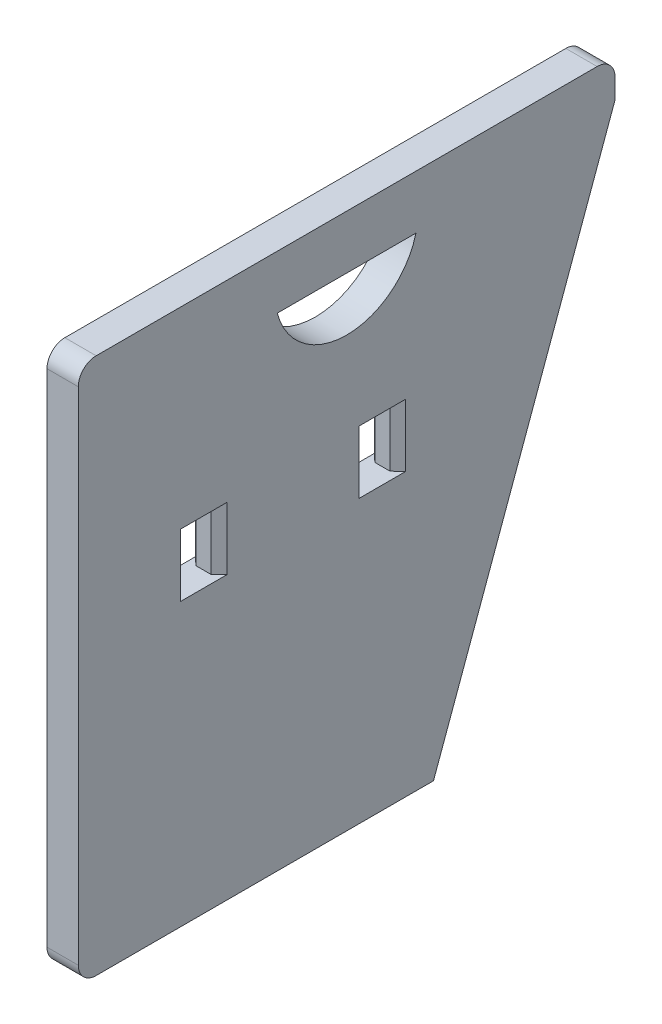
SolidWorks part; units mm, degrees
material "Q235-A"
ref_plane "Front Plane" through (0, 0, 0) normal (0, 0, 1) x (1, 0, 0)
ref_plane "Top Plane" through (0, 0, 0) normal (0, 1, 0) x (1, 0, 0)
ref_plane "Right Plane" through (0, 0, 0) normal (1, 0, 0) x (0, 0, -1)
sketch "Sketch1" plane through (0, 0, 0) normal (1, 0, 0) x (0, 0, -1)
  line L0 (0, 0) -> (0, 300)
  line L1 (0, 300) -> (600, 300)
  line L2 (600, 300) -> (600, 213.7783)
  line L3 (413, -300) -> (0, -300)
  line L4 (0, -300) -> (0, 0)
  line L5 (600, 213.7783) -> (413, -300)
  line L6 (222.5403, 240) -> (377.4597, 240)
  line L7 (0, 0) -> (273.4876, 0) construction
  arc A0 (222.5403, 240) -> (377.4597, 240) centre (300, 260) ccw
  dimension "D1" = 80
  dimension "D2" = 20
  dimension "D3" = 300
  dimension "D4" = 60
  dimension "D5" = 600
  dimension "D6" = 600
  dimension "D7" = 413
  dimension "D8" = 20
extrude "Boss-Extrude1" add sketch "Sketch1" along normal mid plane 35
sketch "Sketch2" plane through (0, 0, 0) normal (0, 1, 0) x (1, 0, 0)
  line L0 (0, 0) -> (0, 459.4565) construction
  line L1 (-17.5, 114) -> (-8.5, 122.5)
  line L2 (-17.5, 600) -> (-17.5, 0) construction
  line L3 (-8.5, 122.5) -> (8.5, 122.5)
  line L4 (8.5, 122.5) -> (17.5, 114)
  line L5 (17.5, 600) -> (17.5, 0) construction
  line L6 (-31.4532, 140) -> (29.3887, 140) construction
  line L7 (17.5, 0) -> (-17.5, 0) construction
  line L8 (8.5, 157.5) -> (17.5, 166)
  line L9 (-8.5, 157.5) -> (8.5, 157.5)
  line L10 (-17.5, 166) -> (-8.5, 157.5)
  line L11 (-17.5, 114) -> (-17.5, 166)
  line L12 (17.5, 114) -> (17.5, 166)
  line L13 (-45.5296, 240) -> (49.3537, 240) construction
  line L14 (8.5, 357.5) -> (17.5, 366)
  line L15 (17.5, 366) -> (17.5, 314)
  line L16 (8.5, 322.5) -> (17.5, 314)
  line L17 (-31.4532, 340) -> (29.3887, 340) construction
  line L18 (-17.5, 314) -> (-8.5, 322.5)
  line L19 (-8.5, 322.5) -> (8.5, 322.5)
  line L20 (-8.5, 357.5) -> (8.5, 357.5)
  line L21 (-17.5, 366) -> (-8.5, 357.5)
  line L22 (-17.5, 366) -> (-17.5, 314)
  dimension "D1" = 140
  dimension "D2" = 35
  dimension "D3" = 52
  dimension "D4" = 17
  dimension "D5" = 100
extrude "Cut-Extrude1" cut sketch "Sketch2" against normal mid plane 70 from offset 50
fillet "Fillet1" radius 20 3 edges at (0, 300, -600) (0, -300, 0) (0, 300, 0)
chamfer "Chamfer2" distance 15 angle 45 1 edges at (17.5, -43.1109, -506.5)
